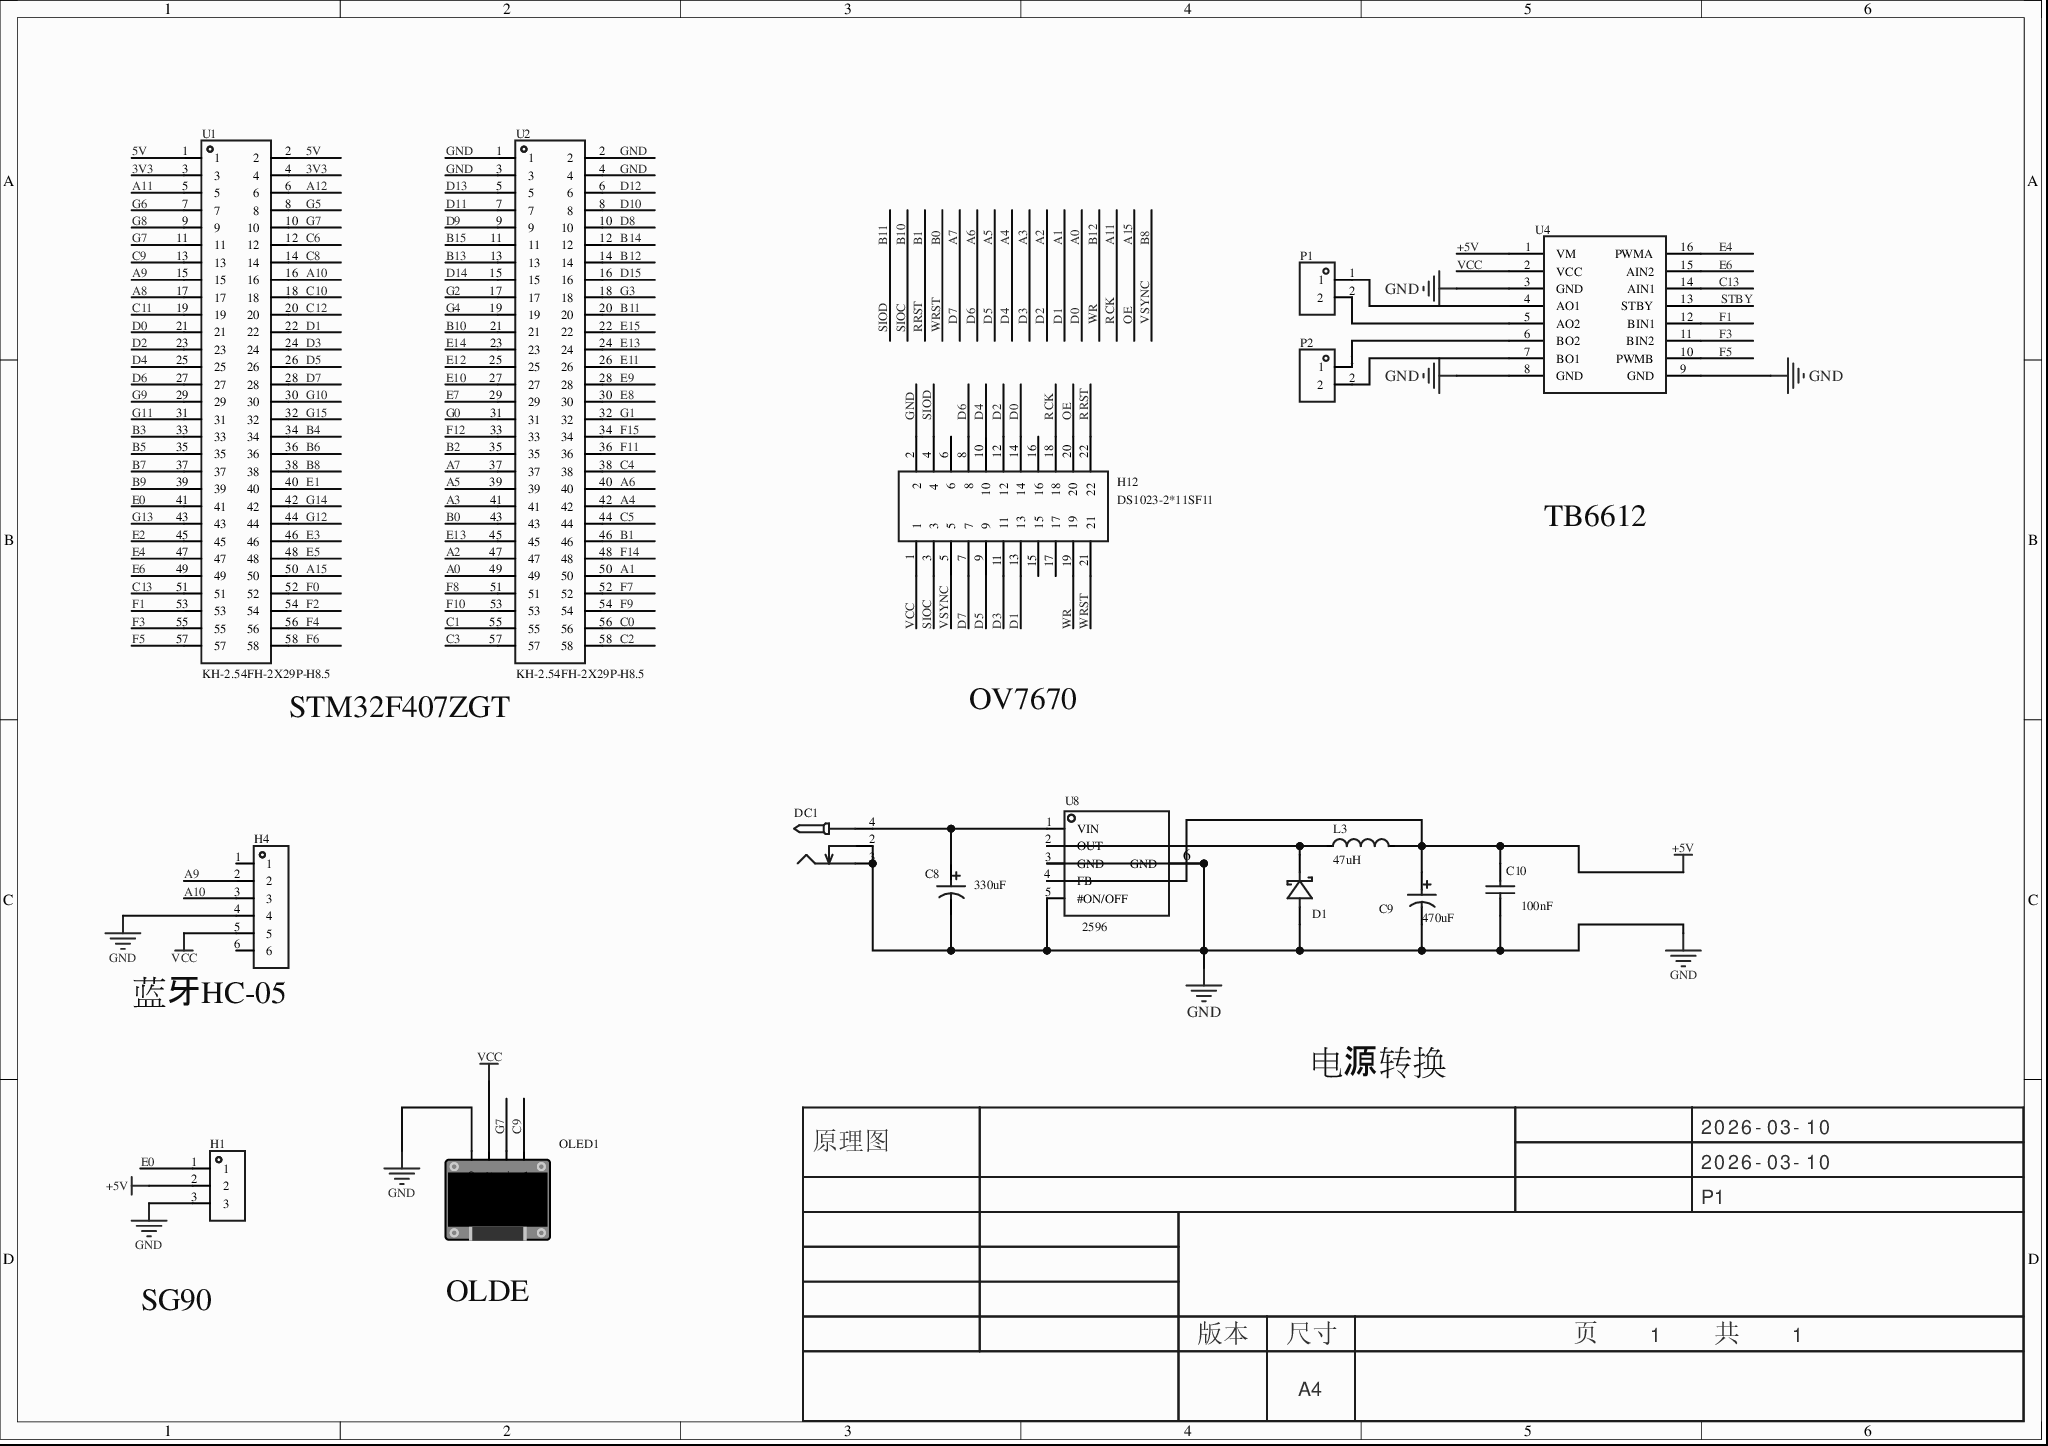
[diagram p0: MISC51443-3.schdoc]
# Altium project MISC51443-2.PrjPcb
1 sheet, 16 parts. Net scope: global (net labels, ports and power ports of the same name join across sheets).
Board file: MISC51443.pcbdoc

## Sheet MISC51443-3.schdoc
size 297 x 209 mm; Version: V1.0; @Project Name: MISC51443; @Update Date: 2026-03-10; @Create Date: 2026-03-10; @Board Name: MISC51443; @Create Time: 20:26:36; @Page Count: 1; @Page No: 1; @Schematic Name: MISC51443; @Update Time: 20:26:36; Size: A4

### Parts
C8  value 330uF  [CAP-SMD_BD8.0-L8.3-W8.3-RD]
C9  value 470uF  [CAP-SMD_BD8.0-L8.3-W8.3-RD]
C10  value 100nF  [C0805]
D1  (no value)  [SMA_L4.3-W2.6-LS5.2-RD]
DC1  (no value)  [DC-2.0]
H1  (no value)  [HDR-TH_3P-P2.54-V-M]
H4  (no value)  [HDR-TH_6P-P2.54-V-F]
H12  DS1023-2*11SF11  [HDR-TH_22P-P2.54-V-F-R2-C11-S2.54]
L3  value 47uH  [IND-SMD_L7.0-W6.6]
OLED1  (no value)  [0.96OLED_4P]
P1  KF301-2P接线端子  [CONN-TH_XY301V-A-5.0-2P]  (value not drawn)
P2  KF301-2P接线端子  [CONN-TH_XY301V-A-5.0-2P]  (value not drawn)
U1  KH-2.54FH-2X29P-H8.5  [HDR-TH_58P-P2.54-V-F-R2-C29-S2.54]
U2  KH-2.54FH-2X29P-H8.5  [HDR-TH_58P-P2.54-V-F-R2-C29-S2.54]
U4  (no value)  [tb6612]
U8  LM2596S-5.0  [TO-263-5_L10.2-W8.9-P1.70-BR]  (value not drawn)

### Nets
+5V: C9.1 C10.1 H1.2 L3.2 U4.1(VM) U8.4(FB)
GND: C8.2 C9.2 C10.2 D1.2(A) DC1.2 DC1.3 H1.3 H4.4 H12.2 OLED1.1(GND) U2.1 U2.2 U2.3 U2.4 U4.3(GND) U4.8(GND) U4.9(GND) U8.3(GND) U8.5(#ON/OFF) U8.6(GND)
VCC: H4.5 H12.1 OLED1.2(VCC) U4.2(VCC)
3V3: U1.3 U1.4
5V: U1.1 U1.2
A0: H12.14 U1.21 U2.49  [also labelled D0]
A1: H12.13 U1.22 U2.50  [also labelled D1]
A2: H12.12 U1.23 U2.47  [also labelled D2]
A3: H12.11 U1.24 U2.41  [also labelled D3]
A4: H12.10 U1.25 U2.42  [also labelled D4]
A5: H12.9 U1.26 U2.39  [also labelled D5]
A6: H12.8 U1.27 U2.40  [also labelled D6]
A7: H12.7 U1.28 U2.37  [also labelled D7]
A8: U1.17
A9: H4.2 U1.15
A10: H4.3 U1.16
A11: H12.18 U1.5  [also labelled RCK]
A12: U1.6
A15: H12.20 U1.50  [also labelled OE]
B0: H12.21 U2.43  [also labelled WRST]
B1: H12.22 U2.46  [also labelled RRST]
B2: U2.35
B3: U1.33
B4: U1.34
B5: U1.35
B6: U1.36
B7: U1.37
B8: H12.5 U1.38  [also labelled VSYNC]
B9: U1.39
B10: H12.3 U2.21  [also labelled SIOC]
B11: H12.4 U2.20  [also labelled SIOD]
B12: H12.19 U2.14  [also labelled WR]
B13: U2.13
B14: U2.12
B15: U2.11
C0: U2.56
C1: U2.55
C2: U2.58
C3: U2.57
C4: U2.38
C5: U2.44
C6: U1.12
C8: U1.14
C9: OLED1.4(SDA) U1.13
C10: U1.18
C11: U1.19
C12: U1.20
C13: U1.51 U4.14(AIN1)
D8: U2.10
D9: U2.9
D10: U2.8
D11: U2.7
D12: U2.6
D13: U2.5
D14: U2.15
D15: U2.16
E0: H1.1 U1.41
E1: U1.40
E2: U1.45
E3: U1.46
E4: U1.47 U4.16(PWMA)
E5: U1.48
E6: U1.49 U4.15(AIN2)
E7: U2.29
E8: U2.30
E9: U2.28
E10: U2.27
E11: U2.26
E12: U2.25
E13: U2.24 U2.45
E14: U2.23
E15: U2.22
F0: U1.52
F1: U1.53 U4.12(BIN1)
F2: U1.54
F3: U1.55 U4.11(BIN2)
F4: U1.56
F5: U1.57 U4.10(PWMB)
F6: U1.58
F7: U2.52
F8: U2.51
F9: U2.54
F10: U2.53
F11: U2.36
F12: U2.33
F14: U2.48
F15: U2.34
G0: U2.31
G1: U2.32
G2: U2.17
G3: U2.18
G4: U2.19
G5: U1.8
G6: U1.7
G7: OLED1.3(SCL) U1.10 U1.11
G8: U1.9
G9: U1.29
G10: U1.30
G11: U1.31
G12: U1.44
G13: U1.43
G14: U1.42
G15: U1.32
STBY: U4.13(STBY)
NetC8_1: C8.1 DC1.4 U8.1(VIN)
NetD1_1: D1.1(K) L3.1 U8.2(OUT)
NetP1_1: P1.1 U4.4(AO1)
NetP1_2: P1.2 U4.5(AO2)
NetP2_1: P2.1 U4.6(BO2)
NetP2_2: P2.2 U4.7(BO1)

Not connected (* = marked no-connect by the designer): H4 1 6; H12 6* 15* 16* 17*

### Notes on the sheet
- TB6612
- STM32F407ZGT
- OV7670
- (near H4) 蓝牙HC-05
- 电源转换
- OLDE
- SG90
- 2026-03-10
- 原理图
- P1
- 版本
- 尺寸
- A4
- 页    1    共    1

### Library data of the parts
C8 C9 = CS1V221M-CRF10　: 容值:220uF;精度:±20%;额定电压:35V;电容体直径:8mm;电容体长度:10.5mm;纹波电流:-;等效串联电阻:-;工作寿命:2000hrs@105;工作温度:-40~+105;; Manufacturer: ST(先科); Rated Voltage: 25V; 3D Model: b102f1362be24624a1b1334fec8dc7f4; 3D Model Transform: 354.33,326.81037,0,0,0,0,0,0,0; Tolerance: ±20%; φD: 8mm; L: 10.5mm; AddInBom: yes; Symbol: CS1V221M-CRF10; Device: CS1V221M-CRF10; Lifetime @ Temp: 2000hrs@105; Operating Temperature: -40~+105; Manufacturer Part: CS1V221M-CRF10; Supplier Footprint: SMD,8x10.5mm; JLCPCB Part Class: Extended Part; Datasheet: https://atta.szlcsc.com/upload/public/pdf/source/20170325/1490427945143.pdf; Supplier: LCSC; Ripple Current: -; Equivalent Series Resistance(ESR): -; ConvertToPcb: yes; FootprintName: CAP-SMD_BD8.0-L8.3-W8.3-RD; ModelName: CAP-SMD_BD8.0-L8.3-W8.3-RD
  C8: Supplier Part: C97814
C10 = CL21B104KBCNNNC: 容值:100nF;精度:±10%;额定电压:50V;温度系数:X7R;; Manufacturer: SAMSUNG(三星); 3D Model: 1ba041120af144c991958decab20d241; 3D Model Transform: 78.74,51.181,0,0,0,0,0,0.0005,0; Tolerance: ±10%; Voltage Rated: 50V; Temperature Coefficient: X7R; AddInBom: yes; ModelName: C0805_L2.0-W1.3-H1.3; Symbol: CL21B104KBCNNNC; Device: CL21B104KBCNNNC; LCSC Part Name: 100nF ±10% 50V; Supplier Part: C1711; Manufacturer Part: CL21B104KBCNNNC; Supplier Footprint: 0805; JLCPCB Part Class: Extended Part; Datasheet: https://atta.szlcsc.com/upload/public/pdf/source/20160103/1457707693305.pdf; Supplier: LCSC; ConvertToPcb: yes; FootprintName: C0805
D1 = SS34_3: Manufacturer: TDD(台冠电子); Manufacturer Part: SS34; Symbol: SS34_C3032484; 3D Model: 7ed2c9d0a4a74bbdbba07ab4052caf5b; 3D Model Transform: 185.039,102.362,0,0,0,0,0,0,0; AddInBom: yes; Device: SS34_3; LCSC Part Name: SS34; Supplier Part: C3032484; Supplier Footprint: SMA; JLCPCB Part Class: Extended Part; Datasheet: https://atta.szlcsc.com/upload/public/pdf/source/20220622/9D70D0693761B542BF6F533590093AA5.pdf; Supplier: LCSC; ConvertToPcb: yes; FootprintName: SMA_L4.3-W2.6-LS5.2-RD; ModelName: SMA_L4.3-W2.6-LS5.2-RD
DC1 = DC-005_2.0: Symbol: DC电源接口; ConvertToPcb: yes; ModelId: f5f20b8a2308479b936ba3c2698865bb0819f05c4eef4c71ace90d822a990e87; ModelName: DC-IN-TH_DC-5520-1; ModelTransform: 372.05,551.18,582.68,90,0,0,137.8,0,-149.61; Device: DC-005_2.0; AddInBom: yes; Supplier Footprint: 插件; FootprintName: DC-2.0
H1 = HDR-M_2.54_1x3P: AddInBom: yes; ModelId: bb473b6d38ff42a99216a4fcdbdcc4cb0819f05c4eef4c71ace90d822a990e87; ModelName: HDR-TH_3P-P2.54-M-LI-1X3P; ModelTransform: 300.03877,100,0,0,0,0,0,0,-118.11; Symbol: HDR-M_2.54_1x3P; Device: HDR-M_2.54_1x3P; ConvertToPcb: yes; FootprintName: HDR-TH_3P-P2.54-V-M; SupplierPart: C2937625; Supplier Footprint: 插件
H4 = HDR-F_2.54_1x6P: Symbol: Header-Female-2.54_1x6; 3D Model: 0f5bcf94dcda47d085f24cdca1696fe9; 3D Model Transform: 619.684,94.488,0,0,0,0,0,0,-125.984; ConvertToPcb: yes; Device: HDR-F_2.54_1x6P; Supplier Part: C40877; Supplier Footprint: 插件; AddInBom: yes; FootprintName: HDR-TH_6P-P2.54-V-F; ModelName: HDR-TH_6P-P2.54-V-F
H12 = DS1023-2*11SF11: 插孔结构:2x11P;间距:2.54mm;行距:2.54mm;安装方式:直插;排数:双排;总孔位数:22P;额定电流:3A;额定电压:600V;插孔方向:顶部;塑高:8.5mm;触头材质:-;触头镀层:金;工作温度:-40℃~+105℃;; Manufacturer: CONNFLY; 3D Model: b6ea5501445d4aa39df4728bd1507c09; 3D Model Transform: 1115.7458,196.85,0,0,0,0,0,0,-118.11; Holes Structure: 2x11P; Pitch: 2.54mm; Number of Positions: 22P; Current Rating: 3A; Voltage Rating (Max): 600V; Holes Direction: 顶部; AddInBom: yes; ModelName: HDR-TH_22P-P2.54-F-LI-2X11P; Symbol: DS1023-2*11SF11; Device: DS1023-2*11SF11; LCSC Part Name: 2x11P 间距:2.54mm 直插; Supplier Part: C132126; Manufacturer Part: DS1023-2*11SF11; Supplier Footprint: 插件,P=2.54mm; JLCPCB Part Class: 扩展库; Datasheet: https://item.szlcsc.com/datasheet/DS1023-2*11SF11/143425.html; Supplier: LCSC; Row Spacing: 2.54mm; Mounting Type: 直插; Number of Rows: 双排; Insulation Height: 8.5mm; Contact Material: -; Contact Plating: 金; Operating Temperature: -40℃~+105℃; ConvertToPcb: yes; FootprintName: HDR-TH_22P-P2.54-V-F-R2-C11-S2.54
L3 = CMLO0630H330MTT: 电感值:33uH;精度:±20%;直流电阻(DCR):270mΩ;; Manufacturer: Cybermax(思博科技); 3D Model: 6860c29aec394a38a0f014af7f722a42; 3D Model Transform: 275.6,259.8,0,0,0,0,0,0,0; Tolerance: ±20%; DC Resistance (DCR): 270mΩ; AddInBom: yes; ModelName: IND-SMD_L7.0-W6.6-H3.0; Symbol: CMLO0630H330MTT; Device: CMLO0630H330MTT; LCSC Part Name: 33uH ±20% 270mΩ; Manufacturer Part: CMLO0630H330MTT; Supplier Footprint: SMD; JLCPCB Part Class: Extended Part; Datasheet: https://atta.szlcsc.com/upload/public/pdf/source/20201124/C961478_55C23F293F63DC1D2CF3D7AB16D0E182.pdf; Supplier: LCSC; ConvertToPcb: yes; FootprintName: IND-SMD_L7.0-W6.6
OLED1 = 0.96OLED模块_4P: ConvertToPcb: yes; ModelId: 79c000fdb68d45a296c2e9bedf4f90550819f05c4eef4c71ace90d822a990e87; ModelTransform: 1393.69792,1318.895,0,0,0,0,0,-560.079,-137.795; Symbol: 0.96OLED模块_4P; Device: 0.96OLED模块_4P; AddInBom: yes; FootprintName: 0.96OLED_4P; Supplier Footprint: 插件; ModelName: 0.96OLED_4P
P1 P2 = KF301-2P接线端子: 3D Model: ef7ead88b0f2448d904975b26718870f; 3D Model Transform: 417.322,299.212,0,0,0,0,11.811,-7.835,-157.48; AddInBom: yes; Symbol: KF301-2P接线端子; Device: KF301-2P接线端子; LCSC Part Name: KF301-2P接线端子; Supplier Part: C9900016950; Manufacturer Part: KF301-2P接线端子; Supplier Footprint: CK301-2P; Supplier: LCSC; ConvertToPcb: yes; FootprintName: CONN-TH_XY301V-A-5.0-2P; ModelName: CONN-TH_XY301V-A-5.0-2P
U1 U2 = KH-2.54FH-2X29P-H8.5: 2.54FH H8.5 2x29Pin 180度 Y型 PC3.2 6T; Manufacturer: kinghelm(金航标); AddInBom: yes; ModelId: 22cfdafb575849e1b4f2e6914e1be6060819f05c4eef4c71ace90d822a990e87; ModelName: HDR-TH_58P-P2.54-F-LI-2X29P; ModelTransform: 2899.99436,200,0,0,0,0,0,0,-118.11; Symbol: KH-2.54FH-2X29P-H8.5; Device: KH-2.54FH-2X29P-H8.5; LCSC Part Name: KH-2.54FH-2X29P-H8.5; SupplierPart: C22440851; ManufacturerPart: KH-2.54FH-2X29P-H8.5; Supplier Footprint: 插件,P=2.54mm; JLCPCB Part Class: Extended Part; Datasheet: https://atta.szlcsc.com/upload/public/pdf/source/20240528/459183379467C01D8D10E0D8CB43AC9D.pdf; Supplier: LCSC; ConvertToPcb: yes; FootprintName: HDR-TH_58P-P2.54-V-F-R2-C29-S2.54
U4 = tb6612: AddInBom: yes; Symbol: tb6612; Device: tb6612; JLCPCB Part Class: 扩展库; ConvertToPcb: yes; FootprintName: tb6612
U8 = LM2596S-5.0_C347421: 功能类型:降压型;输出类型:固定;输入电压:40V;输出电压:5V;输出电流(最大值):3A;; Manufacturer: UMW(广东友台半导体); Symbol: LM2596-TO263; Add into BOM: yes; 3D Model: 4e421a816a7f4d57b8710832ddea550a; 3D Model Transform: 401.574,560.17797,0,90,0,0,-45.276,0,0; Function: 降压型; Synchronous Rectification: 否; Output Type: 固定; Number of Outputs: 1; Topology: 降压式; Input Voltage: 40V; Output Voltage: 5V; Output Current (Max): 3A; Switching Frequency: 150kHz; ModelName: TO-263-5-5P_L10.2-W8.7-H4.5-LS14.4-P1.70; Device: LM2596S-5.0_C347421; Convert to PCB: yes; LCSC Part Name: 降压型 输入40V 输出5V 3A; Supplier Part: C347421; Manufacturer Part: LM2596S-5.0; Supplier Footprint: TO-263-5; JLCPCB Part Class: Extended Part; Datasheet: https://atta.szlcsc.com/upload/public/pdf/source/20211011/C7416AEF3194BD283261B8F2553C4145.pdf; Supplier: LCSC; Operating Temperature: -40℃~+125℃@(TA); FootprintName: TO-263-5_L10.2-W8.9-P1.70-BR